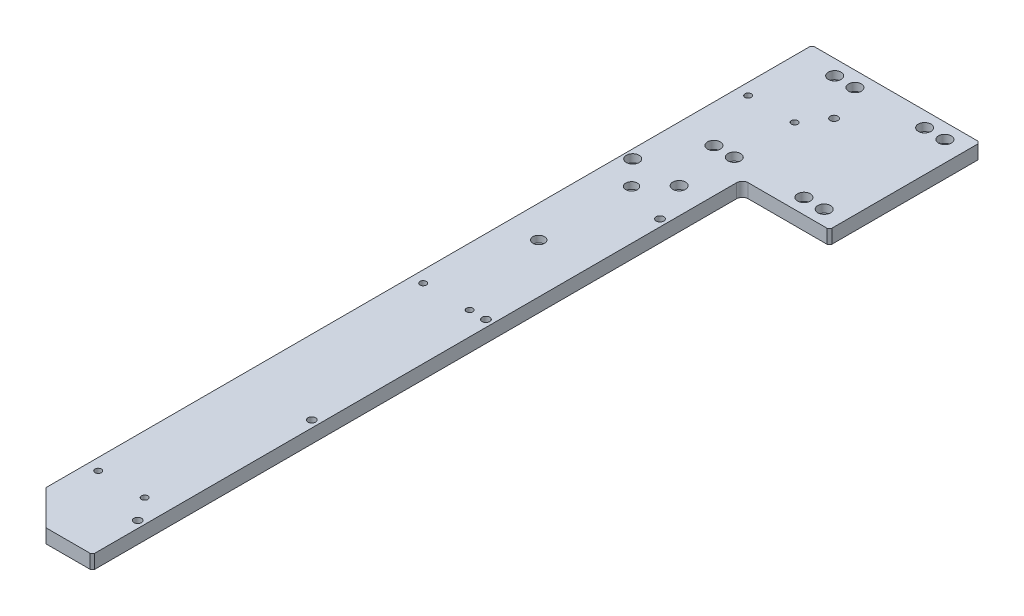
from build123d import *

# Parameters (mm, degrees)
SKETCH_1_W                = 145
SKETCH_1_H                = 690
EXTRUDE_1_DEPTH           = 6
CUT_EXTRUDE_1_DEPTH       = 353.739634858
CHAMFER_1_SIZE            = 2
HOLE_WIZARD_1_D           = 6.6
HOLE_WIZARD_1_CBORE_D     = 11
HOLE_WIZARD_1_CBORE_DEPTH = 6.8
HOLE_WIZARD_2_D           = 6.6
HOLE_WIZARD_2_CBORE_D     = 11
HOLE_WIZARD_2_CBORE_DEPTH = 6.8
HOLE_WIZARD_3_D           = 5.5
HOLE_WIZARD_3_CBORE_D     = 10
HOLE_WIZARD_3_CBORE_DEPTH = 5.7
HOLE_WIZARD_M5_1_D        = 4.2
HOLE_WIZARD_M5_1_DEPTH    = 12.4
HOLE_WIZARD_M5_1_TIP      = 1.2618073
HOLE_WIZARD_4_D           = 6.6
HOLE_WIZARD_4_CBORE_D     = 11
HOLE_WIZARD_4_CBORE_DEPTH = 6.8
HOLE_WIZARD_5_D           = 5.5
HOLE_WIZARD_5_CBORE_D     = 10
HOLE_WIZARD_5_CBORE_DEPTH = 5.7
CHAMFER_2_SIZE            = 30


with BuildPart() as part:
    # 草图1 → 凸台-拉伸1 (new, symmetric)
    with BuildSketch(Plane(origin=(0, 0, 0), x_dir=(1, 0, 0), z_dir=(0, 1, 0))):
        Rectangle(SKETCH_1_W, SKETCH_1_H)
    extrude(amount=EXTRUDE_1_DEPTH, both=True)

    # 草图2 → 切除-拉伸1 (cut, through all)
    with BuildSketch(Plane(origin=(0, 6, 0), x_dir=(1, 0, 0), z_dir=(0, 1, 0))):
        with BuildLine():
            Line((72.5, -345), (-2.5, -345))
            Line((-2.5, -345), (-2.5, 210))
            ThreePointArc((-2.5, 210), (-1.035533906, 213.535533906), (2.5, 215))
            Line((2.5, 215), (72.5, 215))
            Line((72.5, 215), (72.5, -345))
        make_face()
    extrude(amount=-CUT_EXTRUDE_1_DEPTH, mode=Mode.SUBTRACT)

    # 倒角1
    chamfer_1_edges = [part.edges().sort_by_distance(p)[0] for p in [
        (72.5, 0, -215),
        (-2.5, 0, 345),
        (-72.5, 0, -345),
        (72.5, 0, -345),
    ]]
    chamfer(chamfer_1_edges, length=CHAMFER_1_SIZE)

    # 打孔尺寸(%根据)内六角圆柱头螺钉的类型1 (through all)
    with Locations(Plane(origin=(0, 6, 0), x_dir=(1, 0, 0), z_dir=(0, 1, 0))):
        with Locations((-40, 228), (-22.5, 228), (37.5, 228), (55, 228), (55, 332), (37.5, 332), (-22.5, 332), (-40, 332)):
            CounterBoreHole(HOLE_WIZARD_1_D / 2, HOLE_WIZARD_1_CBORE_D / 2, HOLE_WIZARD_1_CBORE_DEPTH)

    # 打孔尺寸(%根据)内六角圆柱头螺钉的类型2 (through all)
    with Locations(Plane(origin=(0, -6, 0), x_dir=(-1, 0, 0), z_dir=(0, -1, 0))):
        with Locations((8.5, 300), (8.5, 150), (8.5, 0), (8.5, -150), (8.5, -300)):
            CounterBoreHole(HOLE_WIZARD_2_D / 2, HOLE_WIZARD_2_CBORE_D / 2, HOLE_WIZARD_2_CBORE_DEPTH)

    # 打孔尺寸(%根据)内六角圆柱头螺钉的类型3 (through all)
    with Locations(Plane(origin=(0, -6, 0), x_dir=(-1, 0, 0), z_dir=(0, -1, 0))):
        with Locations((22.5, 280), (62.5, 280), (22.5, 0), (62.5, 0), (22.5, -280), (62.5, -280)):
            CounterBoreHole(HOLE_WIZARD_3_D / 2, HOLE_WIZARD_3_CBORE_D / 2, HOLE_WIZARD_3_CBORE_DEPTH)

    # M5 螺纹孔1
    with Locations(Plane(origin=(0, 0, -345), x_dir=(-1, 0, 0), z_dir=(0, 0, -1))):
        with Locations((-7.5, 0), (-47.5, 0)):
            Hole(HOLE_WIZARD_M5_1_D / 2, depth=HOLE_WIZARD_M5_1_DEPTH)
            with Locations((0, 0, -(HOLE_WIZARD_M5_1_DEPTH + HOLE_WIZARD_M5_1_TIP / 2))):  # 118° drill point
                Cone(0, HOLE_WIZARD_M5_1_D / 2, HOLE_WIZARD_M5_1_TIP, mode=Mode.SUBTRACT)

    # 打孔尺寸(%根据)内六角圆柱头螺钉的类型4 (through all)
    with Locations(Plane(origin=(0, 6, 0), x_dir=(1, 0, 0), z_dir=(0, 1, 0))):
        with Locations((-65, 183), (-25, 183)):
            CounterBoreHole(HOLE_WIZARD_4_D / 2, HOLE_WIZARD_4_CBORE_D / 2, HOLE_WIZARD_4_CBORE_DEPTH)

    # 打孔尺寸(%根据)内六角圆柱头螺钉的类型5 (through all)
    with Locations(Plane(origin=(0, 6, 0), x_dir=(1, 0, 0), z_dir=(0, 1, 0))):
        with Locations((-45, 162), (-45, 82)):
            CounterBoreHole(HOLE_WIZARD_5_D / 2, HOLE_WIZARD_5_CBORE_D / 2, HOLE_WIZARD_5_CBORE_DEPTH)

    # 倒角2
    chamfer_2_edges = [part.edges().sort_by_distance(p)[0] for p in [
        (-72.5, 0, 345),
    ]]
    chamfer(chamfer_2_edges, length=CHAMFER_2_SIZE)


solid = part.part
